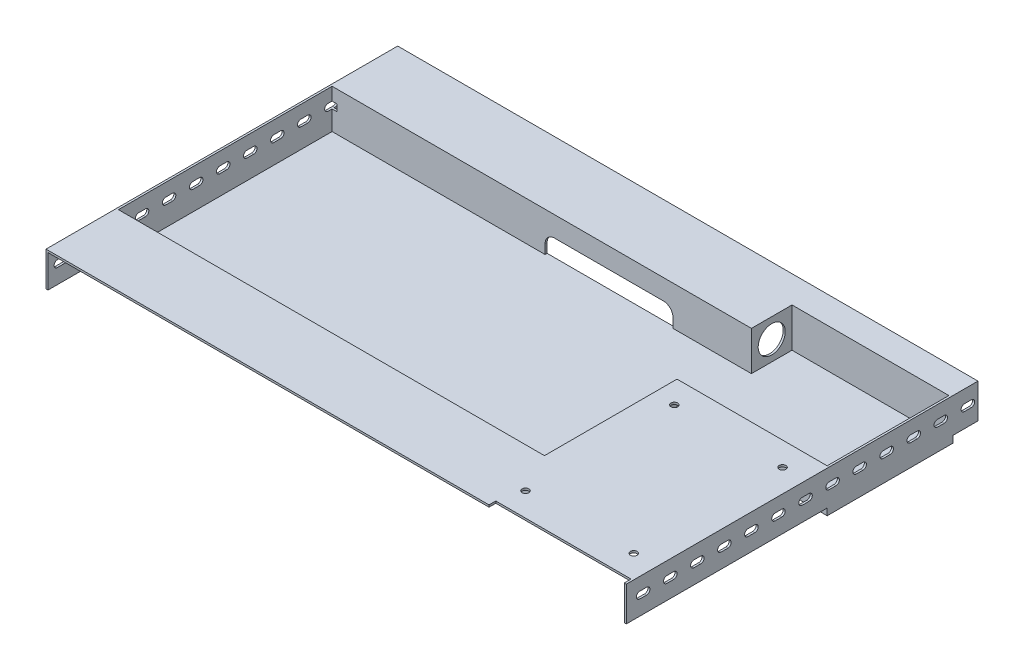
from build123d import *

# Parameters (mm, degrees)
SKETCH_1_W             = 429
SKETCH_1_H             = 260
EXTRUDE_1_DEPTH        = 1.5
CUT_EXTRUDE_1_DEPTH    = 1.5
EXTRUDE_6_DEPTH        = 27.5
EXTRUDE_7_DEPTH        = 1.5
SKETCH_10_W            = 1.5
SKETCH_10_H            = 260
EXTRUDE_8_DEPTH        = 24
CUT_EXTRUDE_2_DEPTH    = 5
CUT_EXTRUDE_3_DEPTH    = 5
PATTERN_LINEAR_1_COUNT = 13
PATTERN_LINEAR_1_PITCH = 20
PATTERN_LINEAR_2_COUNT = 13
PATTERN_LINEAR_2_PITCH = 20
SKETCH_13_W            = 100
SKETCH_13_H            = 5
CUT_EXTRUDE_4_DEPTH    = 5
SKETCH_19_R            = 10
CUT_EXTRUDE_9_DEPTH    = 1.5
CUT_EXTRUDE_10_DEPTH   = 10
SKETCH_21_W            = 81
SKETCH_21_H            = 25
CUT_EXTRUDE_11_DEPTH   = 503.564672455
SKETCH_22_W            = 78
SKETCH_22_H            = 1.5
EXTRUDE_10_DEPTH       = 29
SKETCH_23_W            = 81
SKETCH_23_H            = 25
EXTRUDE_11_DEPTH       = 1.5
SKETCH_24_R            = 2.5
CUT_EXTRUDE_12_DEPTH   = 1.5
SKETCH_25_W            = 94.5
SKETCH_25_H            = 7
CUT_EXTRUDE_13_DEPTH   = 10


with BuildPart() as part:
    # 草图1 → 凸台-拉伸1 (new body)
    with BuildSketch(Plane(origin=(0, 0, 0), x_dir=(1, 0, 0), z_dir=(0, 1, 0))):
        with Locations((214.5, 130)):
            Rectangle(SKETCH_1_W, SKETCH_1_H)
    extrude(amount=EXTRUDE_1_DEPTH)

    # 草图2 → 切除-拉伸1 (cut)
    with BuildSketch(Plane(origin=(0, 1.5, 0), x_dir=(1, 0, 0), z_dir=(0, 1, 0))):
        Polygon((311.5, 210), (311.5, 240), (427.5, 240), (427.5, 150), (397.5, 150), (397.5, 175), (316.5, 175), (316.5, 52), (1.5, 52), (1.5, 210), align=None)
    extrude(amount=-CUT_EXTRUDE_1_DEPTH, mode=Mode.SUBTRACT)

    # 草图7 → 凸台-拉伸6 (add)
    with BuildSketch(Plane.XZ):
        Polygon((0, -50.5), (318, -50.5), (318, -173.5), (396, -173.5), (396, -148.5), (429, -148.5), (429, -241.5), (310, -241.5), (310, -211.5), (0, -211.5), align=None)
        Polygon((1.5, -52), (316.5, -52), (316.5, -175), (397.5, -175), (397.5, -150), (427.5, -150), (427.5, -240), (311.5, -240), (311.5, -210), (1.5, -210), align=None, mode=Mode.SUBTRACT)
    extrude(amount=EXTRUDE_6_DEPTH)

    # 草图9 → 凸台-拉伸7 (add)
    with BuildSketch(Plane.XZ.offset(27.5)):
        Polygon((318, -50.5), (0, -50.5), (0, -211.5), (310, -211.5), (310, -241.5), (429, -241.5), (429, -148.5), (396, -148.5), (396, -173.5), (318, -173.5), align=None)
    extrude(amount=EXTRUDE_7_DEPTH)

    # 草图10 → 凸台-拉伸8 (add)
    with BuildSketch(Plane.XZ):
        with Locations((0.75, -130)):
            Rectangle(SKETCH_10_W, SKETCH_10_H)
        with Locations((428.25, -130)):
            Rectangle(SKETCH_10_W, SKETCH_10_H)
    extrude(amount=EXTRUDE_8_DEPTH)

    # 草图11 → 切除-拉伸2 (cut)
    with BuildSketch(Plane.ZY):
        with BuildLine():
            Line((-252, -8), (-247, -8))
            ThreePointArc((-247, -8), (-244.5, -10.5), (-247, -13))
            Line((-247, -13), (-252, -13))
            ThreePointArc((-252, -13), (-254.5, -10.5), (-252, -8))
        make_face()
    cut_extrude_2 = extrude(amount=-CUT_EXTRUDE_2_DEPTH, mode=Mode.SUBTRACT)

    # 草图12 → 切除-拉伸3 (cut)
    with BuildSketch(Plane(origin=(429, 0, 0), x_dir=(0, 0, -1), z_dir=(1, 0, 0))):
        with BuildLine():
            Line((250, -8), (255, -8))
            ThreePointArc((255, -8), (257.5, -10.5), (255, -13))
            Line((255, -13), (250, -13))
            ThreePointArc((250, -13), (247.5, -10.5), (250, -8))
        make_face()
    cut_extrude_3 = extrude(amount=-CUT_EXTRUDE_3_DEPTH, mode=Mode.SUBTRACT)

    # 阵列(线性)1: 切除-拉伸2 ×13
    with Locations(*[(0, 0, i * PATTERN_LINEAR_1_PITCH) for i in range(1, PATTERN_LINEAR_1_COUNT)]):
        add(cut_extrude_2, mode=Mode.SUBTRACT)

    # 阵列(线性)2: 切除-拉伸3 ×13
    with Locations(*[(0, 0, i * PATTERN_LINEAR_2_PITCH) for i in range(1, PATTERN_LINEAR_2_COUNT)]):
        add(cut_extrude_3, mode=Mode.SUBTRACT)

    # 草图13 → 切除-拉伸4 (cut)
    with BuildSketch(Plane(origin=(0, 1.5, 0), x_dir=(1, 0, 0), z_dir=(0, 1, 0))):
        with Locations((377.5, 2.5)):
            Rectangle(SKETCH_13_W, SKETCH_13_H)
    extrude(amount=-CUT_EXTRUDE_4_DEPTH, mode=Mode.SUBTRACT)

    # 草图19 → 切除-拉伸9 (cut)
    with BuildSketch(Plane(origin=(311.5, 0, 0), x_dir=(0, 0, -1), z_dir=(1, 0, 0))):
        with Locations((225, -13)):
            Circle(SKETCH_19_R)
    extrude(amount=-CUT_EXTRUDE_9_DEPTH, mode=Mode.SUBTRACT)

    # 草图20 → 切除-拉伸10 (cut)
    with BuildSketch(Plane.XY.offset(-210)):
        with BuildLine():
            Line((246.5, -27.5), (166, -27.5))
            ThreePointArc((166, -27.5), (159, -20.5), (166, -13.5))
            Line((166, -13.5), (246.5, -13.5))
            ThreePointArc((246.5, -13.5), (253.5, -20.5), (246.5, -27.5))
        make_face()
    extrude(amount=-CUT_EXTRUDE_10_DEPTH, mode=Mode.SUBTRACT)

    # 草图21 → 切除-拉伸11 (cut, through all)
    with BuildSketch(Plane(origin=(0, 1.5, 0), x_dir=(1, 0, 0), z_dir=(0, 1, 0))):
        with Locations((357, 162.5)):
            Rectangle(SKETCH_21_W, SKETCH_21_H)
    extrude(amount=-CUT_EXTRUDE_11_DEPTH, mode=Mode.SUBTRACT)

    # 草图22 → 凸台-拉伸10 (add)
    with BuildSketch(Plane.XZ.offset(29)):
        with Locations((357, -149.25)):
            Rectangle(SKETCH_22_W, SKETCH_22_H)
    extrude(amount=-EXTRUDE_10_DEPTH)

    # 草图23 → 凸台-拉伸11 (add)
    with BuildSketch(Plane.XZ.offset(29)):
        with Locations((357, -162.5)):
            Rectangle(SKETCH_23_W, SKETCH_23_H)
    extrude(amount=-EXTRUDE_11_DEPTH)

    # 草图24 → 切除-拉伸12 (cut)
    with BuildSketch(Plane(origin=(0, 1.5, 0), x_dir=(1, 0, 0), z_dir=(0, 1, 0))):
        with Locations(Location((332, 132.5, 0), (0, 0, 270))):
            Circle(SKETCH_24_R)
        with Locations(Location((412, 132.5, 0), (0, 0, 90))):
            Circle(SKETCH_24_R)
        with Locations(Location((412, 22.5, 0), (0, 0, 270))):
            Circle(SKETCH_24_R)
        with Locations(Location((332, 22.5, 0), (0, 0, 90))):
            Circle(SKETCH_24_R)
    extrude(amount=-CUT_EXTRUDE_12_DEPTH, mode=Mode.SUBTRACT)

    # 草图25 → 切除-拉伸13 (cut)
    with BuildSketch(Plane.XY.offset(-210)):
        with Locations((206.25, -24)):
            Rectangle(SKETCH_25_W, SKETCH_25_H)
    extrude(amount=-CUT_EXTRUDE_13_DEPTH, mode=Mode.SUBTRACT)


solid = part.part
